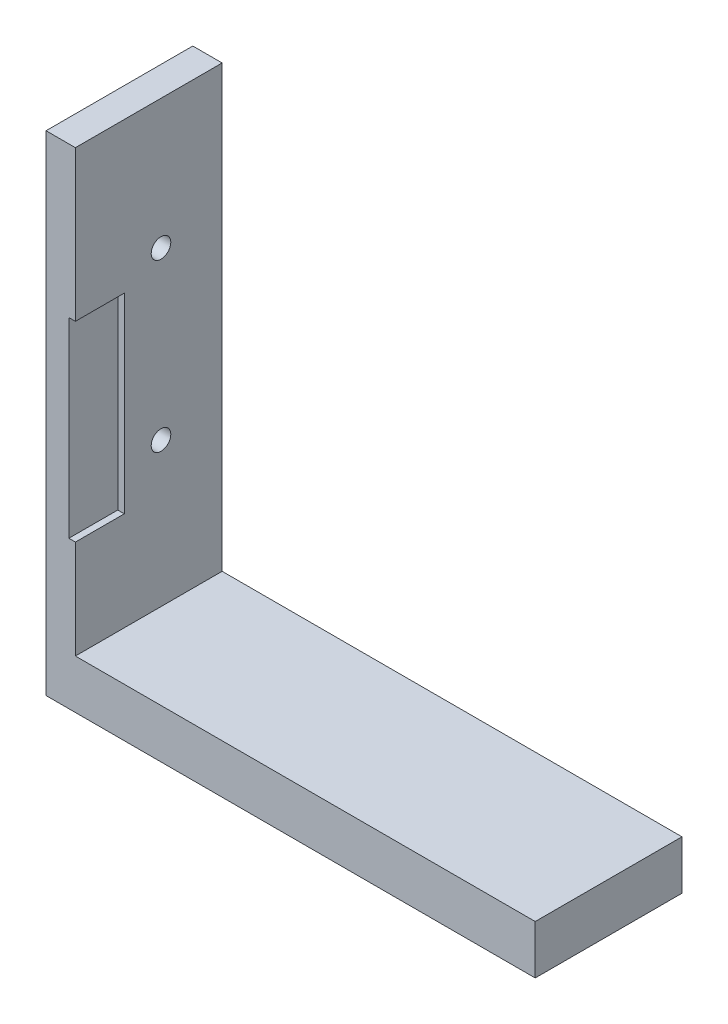
from build123d import *

# Parameters (mm, degrees)
BOSS_EXTRUDE1_DEPTH = 30
SKETCH2_R           = 2
CUT_EXTRUDE1_DEPTH  = 145.568322948
CHAMFER1_SIZE       = 2.1
SKETCH3_W           = 2.678240958
SKETCH3_H           = 39.075972863
CUT_EXTRUDE2_DEPTH  = 10


with BuildPart() as part:
    # Sketch1 → Boss-Extrude1 (new body)
    with BuildSketch(Plane.XY):
        Polygon((0, 0), (100, 0), (100, 10), (6, 10), (6, 100), (0, 100), align=None)
    extrude(amount=BOSS_EXTRUDE1_DEPTH)

    # Sketch2 → Cut-Extrude1 (cut, through all)
    with BuildSketch(Plane.ZY):
        with Locations((12.5, 73.5)):
            Circle(SKETCH2_R)
        with Locations((12.5, 39.5)):
            Circle(SKETCH2_R)
    extrude(amount=-CUT_EXTRUDE1_DEPTH, mode=Mode.SUBTRACT)

    # Chamfer1
    chamfer1_edges = [part.edges().sort_by_distance(p)[0] for p in [
        (0, 73.5, 10.5),
        (0, 39.5, 10.5),
    ]]
    chamfer(chamfer1_edges, length=CHAMFER1_SIZE)

    # Sketch3 → Cut-Extrude2 (cut)
    with BuildSketch(Plane.XY.offset(30)):
        with Locations((6, 49.716029753)):
            Rectangle(SKETCH3_W, SKETCH3_H)
    extrude(amount=-CUT_EXTRUDE2_DEPTH, mode=Mode.SUBTRACT)


solid = part.part
